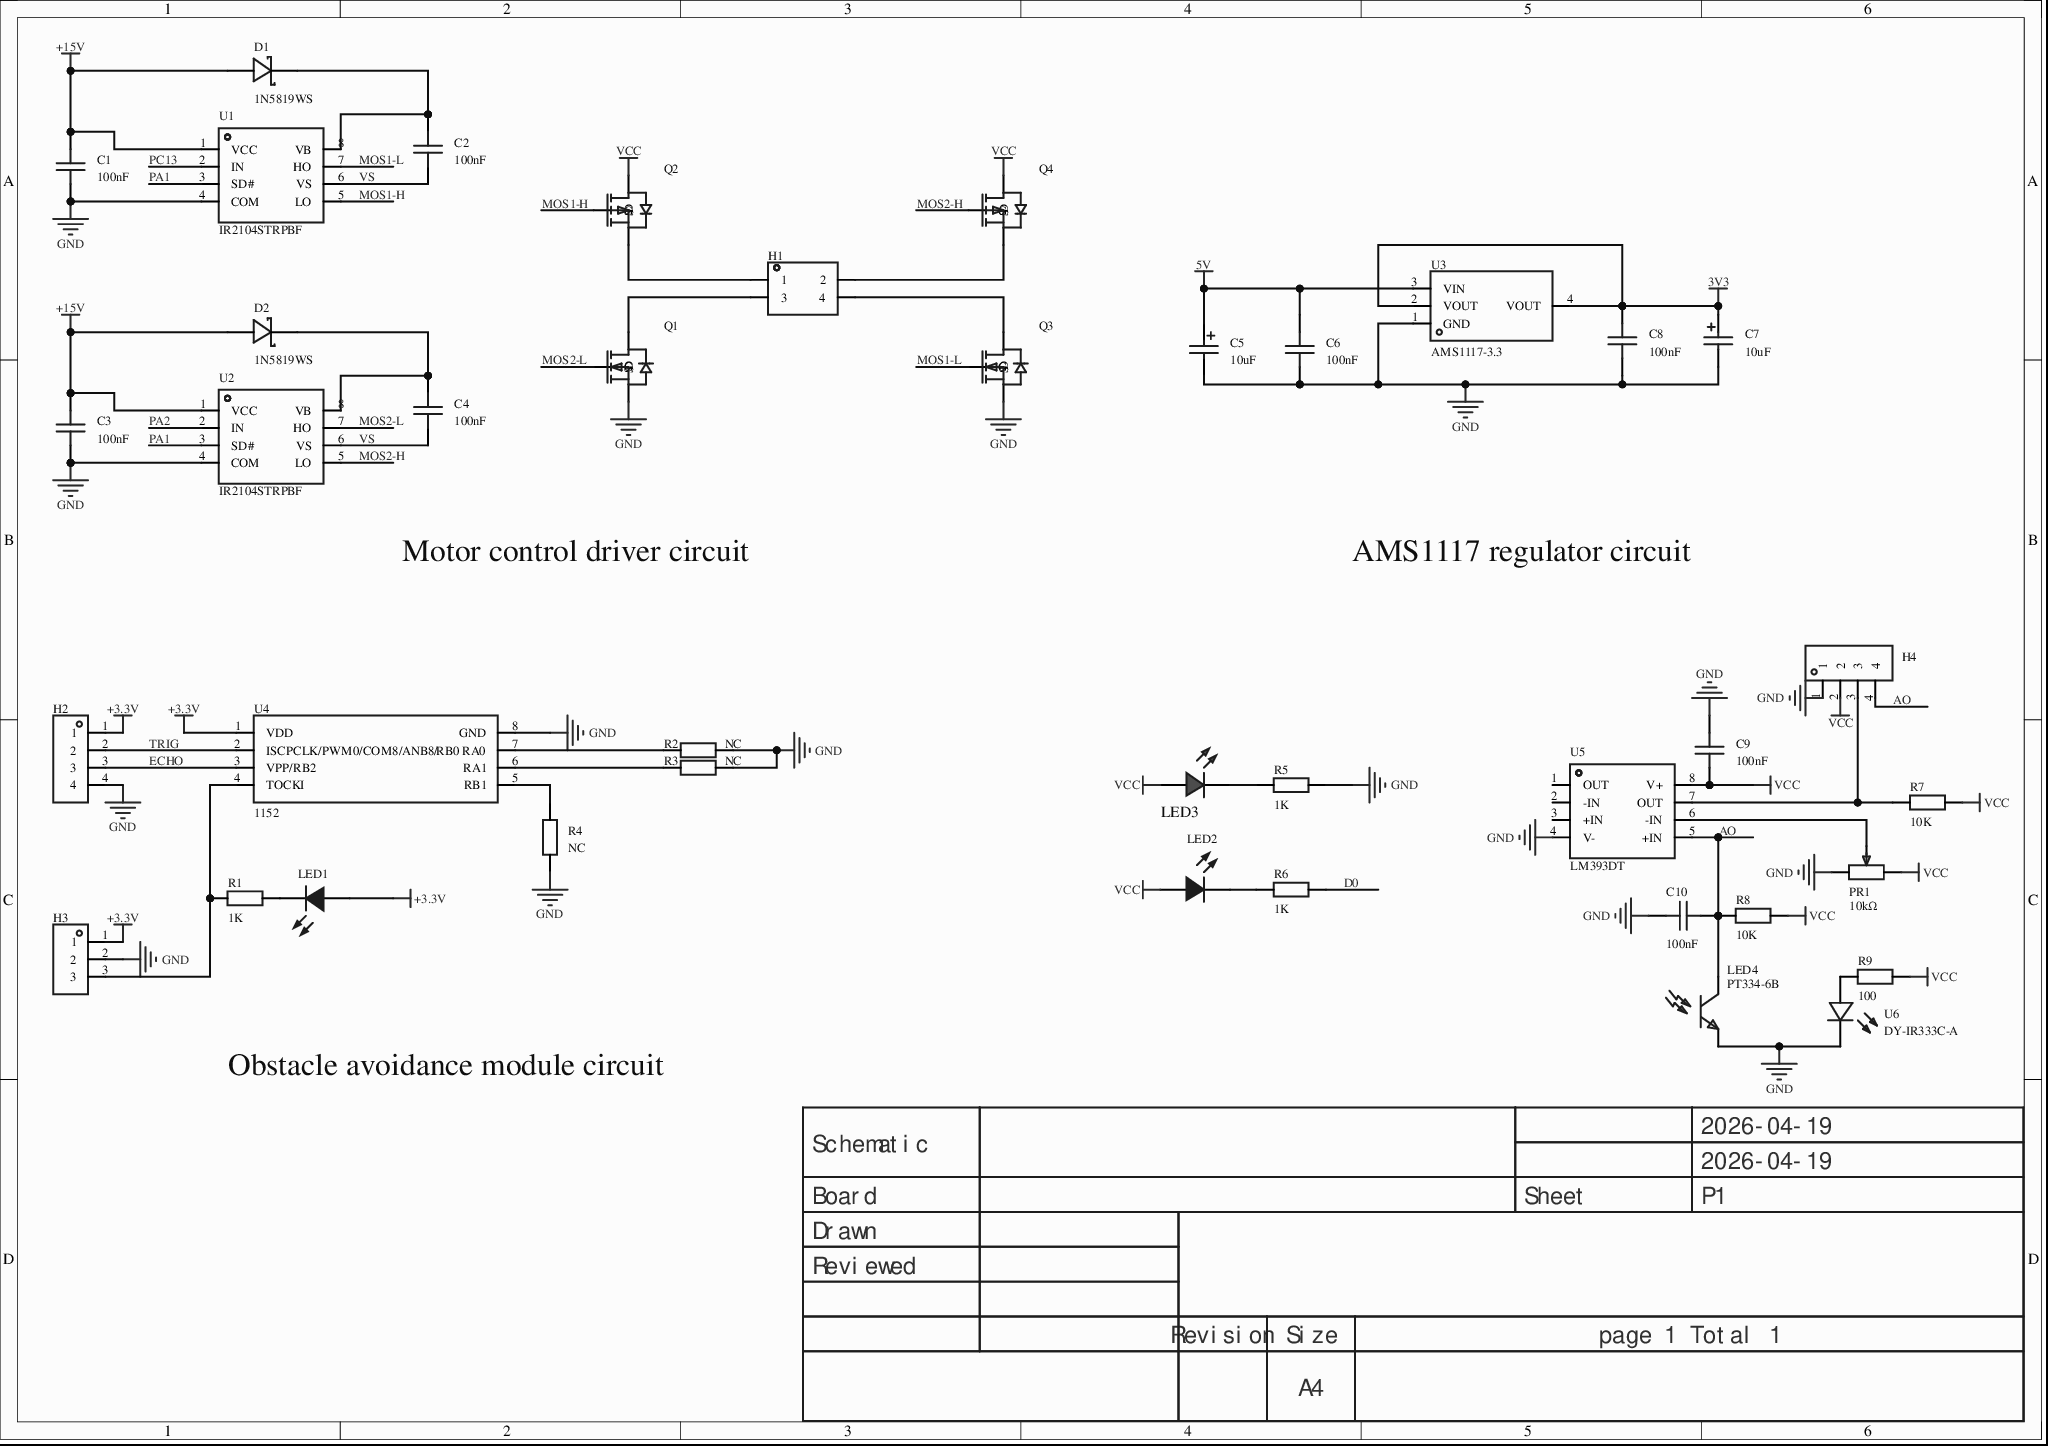
[diagram p0: MISC64784-3.schdoc]
# Altium project MISC64784-2.PrjPcb
1 sheet, 40 parts. Net scope: global (net labels, ports and power ports of the same name join across sheets).
Board file: MISC64784.pcbdoc

## Sheet MISC64784-3.schdoc
size 297 x 209 mm; Version: V1.0; @Project Name: MISC64784; @Update Date: 2026-04-19; @Create Date: 2026-04-19; @Board Name: MISC64784; @Create Time: 10:43:09; @Page Count: 1; @Page No: 1; @Schematic Name: MISC64784; @Update Time: 10:43:09; Size: A4

### Parts
C1  100nF  [C0603]
C2  100nF  [C0603]
C3  100nF  [C0603]
C4  100nF  [C0603]
C5  10uF  [C_Ele_SMD_3x5.4mm]
C6  100nF  [C0603]
C7  10uF  [C_Ele_SMD_3x5.4mm]
C8  100nF  [C0603]
C9  100nF  [C0603]
C10  100nF  [C0603]
D1  1N5819WS  [SOD-323_L1.8-W1.3-LS2.5-RD]
D2  1N5819WS  [SOD-323_L1.8-W1.3-LS2.5-RD]
H1  (no value)  [HDR-TH_4P-P2.54-V-F-R2-C2-S2.54]
H2  (no value)  [HDR-TH_4P-P2.54-V-F]
H3  (no value)  [HDR-TH_3P-P2.54-V-F]
H4  (no value)  [HDR-TH_4P-P2.54-V-M]
LED1  (no value)  [LED_0603]
LED2  (no value)  [LED_0603]
LED3  (no value)  [LED_0603]
LED4  PT334-6B  [LED-TH_BD5.9-P2.54-FD]
PR1  10kΩ  [R_3296]
Q1  (no value)  [SOT-23-3_L2.9-W1.3-P1.90-LS2.4-BR]
Q2  (no value)  [AO3401A_SOT-23-3]
Q3  (no value)  [SOT-23-3_L2.9-W1.3-P1.90-LS2.4-BR]
Q4  (no value)  [AO3401A_SOT-23-3]
R1  1K  [R0603]
R2  NC  [R0603]
R3  NC  [R0603]
R4  NC  [R0603]
R5  1K  [R0603]
R6  1K  [R0603]
R7  10K  [R0603]
R8  10K  [R0603]
R9  100  [R0603]
U1  IR2104STRPBF  [SOIC-8_L4.9-W3.9-P1.27-LS6.0-BL]
U2  IR2104STRPBF  [SOIC-8_L4.9-W3.9-P1.27-LS6.0-BL]
U3  AMS1117-3.3  [SOT-223-3_L6.5-W3.4-P2.30-LS7.0-BR]
U4  1152  [SOP-8_L4.9-W3.9-P1.27-LS6.0-BL]
U5  LM393DT  [SOIC-8_L5.0-W4.0-P1.27-LS6.0-BL]
U6  DY-IR333C-A  [LED-TH_BD5.9-P2.54-FD]

### Nets
3V3: C7.1 C8.2 U3.2(VOUT) U3.4(VOUT)
5V: C5.1 C6.2 U3.3(VIN)
+3.3V: H2.1 H3.1 LED1.2(A) U4.1(VDD)
+15V: C1.2 C3.2 D1.2(A) D2.2(A) U1.1(VCC) U2.1(VCC)
GND: C1.1 C3.1 C5.2 C6.1 C7.2 C8.1 C9.2 C10.1 H2.4 H3.2 H4.1 LED4.1(E) PR1.3 Q1.2(S) Q3.2(S) R2.2 R3.2 R4.2 R5.2 U1.4(COM) U2.4(COM) U3.1(GND) U4.8(GND) U5.4(V-) U6.2(C)
VCC: C9.1 H4.2 LED2.2(A) LED3.2(A) PR1.1 Q2.3(D) Q4.3(D) R7.2 R8.2 R9.2 U5.8(V+)
AO: C10.2 H4.4 LED4.2(C) R8.1 U5.5(+IN)
D0: R6.2
ECHO: H2.3 U4.3(VPP/RB2)
MOS1-H: Q2.1(G) U1.5(LO)
MOS1-L: Q3.1(G) U1.7(HO)
MOS2-H: Q4.1(G) U2.5(LO)
MOS2-L: Q1.1(G) U2.7(HO)
PA1: U1.3(SD#) U2.3(SD#)
PA2: U2.2(IN)
PC13: U1.2(IN)
TRIG: H2.2 U4.2(ISCPCLK/PWM0/COM8/ANB8/RB0)
VS: C2.1 C4.1 U1.6(VS) U2.6(VS)
NetC2_2: C2.2 D1.1(K) U1.8(VB)
NetC4_2: C4.2 D2.1(K) U2.8(VB)
NetH1_1: H1.1 Q2.2(S)
NetH1_2: H1.2 Q4.2(S)
NetH1_3: H1.3 Q1.3(D)
NetH1_4: H1.4 Q3.3(D)
NetH3_3: H3.3 R1.1 U4.4(TOCKI)
NetH4_3: H4.3 R7.1 U5.7(OUT)
NetLED1_1: LED1.1(C) R1.2
NetLED2_1: LED2.1(C) R6.1
NetLED3_1: LED3.1(C) R5.1
NetPR1_2: PR1.2 U5.6(-IN)
NetR2_1: R2.1 U4.7(RA0)
NetR3_1: R3.1 U4.6(RA1)
NetR4_1: R4.1 U4.5(RB1)
NetR9_1: R9.1 U6.1(A)

Not connected (* = marked no-connect by the designer): U5 1(OUT)* 2(-IN)* 3(+IN)*

### Notes on the sheet
- Motor control driver circuit
- AMS1117 regulator circuit
- Obstacle avoidance module circuit
- 2026-04-19
- Schematic
- Board
- Sheet
- P1
- Drawn
- Reviewed
- Revision
- Size
- A4
- page 1 Total 1

### Library data of the parts
C1-C4 C6 C8-C10 = CAP_0603: Symbol: Capacitance; ConvertToPcb: yes; ModelId: ac125912035d415993ca9572d50418b10819f05c4eef4c71ace90d822a990e87; ModelName: C0603_L1.6-W0.8-H0.8; ModelTransform: 62.992,31.496,0,0,0,0,0,0,0; Device: CAP_0603; AddInBom: yes; Supplier Footprint: 0603; FootprintName: C0603; Value: 100nF
C5 C7 = C_Ele_SMD_3x5.4mm: Symbol: CAP; AddInBom: yes; ModelId: 0132c3d3fdbf4fd987f710a97e7a5b5d0819f05c4eef4c71ace90d822a990e87; ModelName: CAP-SMD_BD3.0-L3.3-W3.3-H5.3; ModelTransform: 129.9,149.58,209.06,-90,0,0,0,0,0; Device: C_Ele_SMD_3x5.4mm; Supplier Footprint: SMD,3x5.4mm; ConvertToPcb: yes; FootprintName: C_Ele_SMD_3x5.4mm; Value: 10uF
D1 D2 = 1N5819WS_C191023: Forward voltage drop (Vf): 600mV@1A; DC reverse voltage (Vr): 40V; rectified current: 1A;; Manufacturer: Hottech(合科泰); AddInBom: yes; ModelId: db63db13d9e342eb939127d413d6200b0819f05c4eef4c71ace90d822a990e87; ModelTransform: 104.3305,51.181,0,0,0,0,0,-0.004,0; Non-Repetitive Peak Forward Surge Current: 25A; Symbol: 1N5819WS; Device: 1N5819WS_C191023; LCSC Part Name: 电压:40V 电流:1A; SupplierPart: C191023; ManufacturerPart: 1N5819WS; Supplier Footprint: SOD-323; JLCPCB Part Class: Basic Part; Datasheet: https://example.com/datasheet/1N5819WS/213850.html; Supplier: LCSC; ConvertToPcb: yes; FootprintName: SOD-323_L1.8-W1.3-LS2.5-RD; ModelName: SOD-323_L1.8-W1.3-LS2.5-RD; Voltage - Forward(Vf@If): 600mV@1A; Voltage - DC Reverse(Vr): 40V; Current - Rectified: 1A
H1 = HDR-F_2.54_2x2: Symbol: HDR-F-2.54_2x2; ConvertToPcb: yes; ModelId: 870c884146ee4765973edc845f10b7af0819f05c4eef4c71ace90d822a990e87; ModelName: HDR-TH_4P-P2.54-F-LI-2X2P; ModelTransform: 215.7476,196.85,0,0,0,0,0,0,-118.11; Device: HDR-F_2.54_2x2; AddInBom: yes; SupplierPart: C92273; Supplier Footprint: 插件; FootprintName: HDR-TH_4P-P2.54-V-F-R2-C2-S2.54
H2 = HDR-F_2.54_1x4P: Symbol: 2.54-1*4P female; ConvertToPcb: yes; ModelId: d187812051054f85879fcaa51a310d8e0819f05c4eef4c71ace90d822a990e87; ModelTransform: 419.6842,98.464,0,0,0,0,0,0,-118.11; Device: HDR-F_2.54_1x4P; AddInBom: yes; SupplierPart: C2718488; Supplier Footprint: 插件; FootprintName: HDR-TH_4P-P2.54-V-F; ModelName: HDR-TH_4P-P2.54-V-F
H3 = HDR-F_2.54_1x3P: Symbol: PM254V-11-03-H85; ConvertToPcb: yes; ModelId: f3b3cc5aae9641bf9e56fc160cef875b0819f05c4eef4c71ace90d822a990e87; ModelName: HDR2.54-F-LI-1X3P; ModelTransform: 299.9994,100,0,0,0,0,0,0,-118.11; Device: HDR-F_2.54_1x3P; AddInBom: yes; SupplierPart: C541850; Supplier Footprint: 插件; FootprintName: HDR-TH_3P-P2.54-V-F
H4 = HDR-M_2.54_1x4P: Symbol: PZ254V-11-04P; ConvertToPcb: yes; ModelId: 112f4d05e8d64e99ab9a333894bea4f90819f05c4eef4c71ace90d822a990e87; ModelName: HDR-TH_4P-P2.54-M-LI-1X4P; ModelTransform: 399.999,104.7242,0,0,0,0,0,0,-118.11; Device: HDR-M_2.54_1x4P; AddInBom: yes; SupplierPart: C492403; Supplier Footprint: 插件; FootprintName: HDR-TH_4P-P2.54-V-M
LED1 LED2 = LED_0603-B: Symbol: LED_B; Convert to PCB: yes; 3D Model: eb8d964598f24248affda46f619856c50819f05c4eef4c71ace90d822a990e87; 3D Model Transform: 63.1,31.6,23.7,0,0,0,0,0,0; ModelName: LED-0603_B; Device: LED_0603-B; Add into BOM: yes; Supplier Footprint: 0603; FootprintName: LED_0603
LED3 = LED_0603-R: Symbol: LED_R; Convert to PCB: yes; 3D Model: dd8257b0d61a4cd7b68939a056e080950819f05c4eef4c71ace90d822a990e87; 3D Model Transform: 58.72,29.4,22.03,0,0,0,0,0,0; ModelName: LED-0603_R; Device: LED_0603-R; Add into BOM: yes; Supplier Footprint: 0603; FootprintName: LED_0603
LED4 = PT334-6B: Transistor type: NPN; collector-emitter breakdown voltage (Vceo): 30V; collector current (Ic): 20mA; power dissipation (Pd): 75mW; dark current: 100nA; peak wavelength: 940nm;; Manufacturer: EVERLIGHT(亿光); Symbol: PT334-6B_C369188; AddInBom: yes; ModelId: 002e58ac71644a3881ed56fcedaceeee0819f05c4eef4c71ace90d822a990e87; ModelName: LED-TH_5mm_W; ModelTransform: 214.5665,231.969,0,0,0,0,-9.961,0,-137.795; Vce Saturation(VCE(sat)): 0.4V@2mA; Device: PT334-6B; LCSC Part Name: K档 940nm的NPN光电三极管; SupplierPart: C369188; ManufacturerPart: PT334-6B; Supplier Footprint: 插件,D=5mm; JLCPCB Part Class: Extended Part; Supplier: LCSC; ConvertToPcb: yes; FootprintName: LED-TH_BD5.9-P2.54-FD; type: NPN; Collector - Emitter Voltage VCEO: 30V; Current - Collector(Ic): 20mA; Dissipation Power(Max): 75mW; Current - Dark(Id): 100nA; Peak Wavelength: 940nm; Viewing Angle: -; Operating Temperature: -25℃~+85℃
PR1 = R_3296: ConvertToPcb: yes; ModelId: b182808559bb43bda9e7de64b64134cb0819f05c4eef4c71ace90d822a990e87; ModelName: 3296W; ModelTransform: 373.98,188.96,590.49,180,0,0,0,0,-140; Symbol: R_3296; Device: R_3296; AddInBom: yes; Supplier Footprint: 直插; FootprintName: R_3296; Value: 10kΩ
Q1 Q3 = AO3400A_N: 类型:N沟道;漏源电压(Vdss):30V;连续漏极电流(Id):5.2A;功率(Pd):1W;导通电阻(RDS(on)@Vgs,Id):35mΩ@10V,5A;阈值电压(Vgs(th)@Id):1.5V@250μA;; Symbol: N_MOS; AddInBom: yes; ModelId: c62791f0466c4ae2a892c056b845b0ca0819f05c4eef4c71ace90d822a990e87; ModelName: SOT-23-3P_L2.9-W1.3-H1.0-LS2.4-P0.95; ModelTransform: 98.425,114.173,0,180,0,0,0.0005,-0.0005,0; Device: AO3400A_N; Supplier Footprint: SOT-23; ConvertToPcb: yes; FootprintName: SOT-23-3_L2.9-W1.3-P1.90-LS2.4-BR; SupplierPart: C700953
Q2 Q4 = AO3401A_P: Symbol: P_MOS; AddInBom: yes; ModelId: c62791f0466c4ae2a892c056b845b0ca0819f05c4eef4c71ace90d822a990e87; ModelName: SOT-23-3P_L2.9-W1.3-H1.0-LS2.4-P0.95; ModelTransform: 98.6,114.12,41.29,180,0,0,0,0,0; Device: AO3401A_P; Supplier Footprint: SOT-23-3L; ConvertToPcb: yes; FootprintName: AO3401A_SOT-23-3; SupplierPart: C15127
R1-R9 = Res_0603: Symbol: Resistor; ConvertToPcb: yes; ModelId: fc143cca1e79419f9cd78b61e9279f080819f05c4eef4c71ace90d822a990e87; ModelTransform: 31.8897,63.7794,0,90,0,0,0,0,0; Device: Res_0603; AddInBom: yes; Supplier Footprint: 0603; FootprintName: R0603; ModelName: R0603
  R1 R5 R6: Value: 1K
  R2-R4: Value: NC
  R7 R8: Value: 10K
  R9: Value: 100
U1 U2 = IR2104STRPBF: Driver configuration: half-bridge; load type: IGBT; MOSFET; driver channels: 2; sink current (IOL): 270mA; source current (IOH): 130mA; operating voltage: 10V~20V; rise time (tr): 100ns; fall time (tf): 50ns;; Manufacturer: Infineon(英飞凌); AddInBom: yes; ModelId: e81d2f7d937b4a6ab1dca543ff5d56a40819f05c4eef4c71ace90d822a990e87; ModelName: SOIC-8_L4.9-W3.9-H1.7-LS6.0-P1.27; ModelTransform: 192.913,236.22,0,0,0,0,0,0,0; Number of Drivers: 2; Propagation Delay tpLH: 680ns; Propagation Delay tpHL: 150ns; Quiescent Current(Iq): 150uA; Symbol: IR2104STRPBF; Device: IR2104STRPBF; LCSC Part Name: 半桥驱动器; SupplierPart: C2960; ManufacturerPart: IR2104STRPBF; Supplier Footprint: SOIC-8; JLCPCB Part Class: Extended Part; Datasheet: https://example.com/datasheet/IR2104STRPBF/3342.html; Supplier: LCSC; ConvertToPcb: yes; FootprintName: SOIC-8_L4.9-W3.9-P1.27-LS6.0-BL; Driven Configuration: Half-bridge; Load Type: IGBT; MOSFET; Current - Output Low(IOL): 270mA; Current - Output High(IOH): 130mA; Voltage - Supply: 10V~20V; Rise Time: 100ns; Fall Time: 50ns; Features: Undervoltage protection (UVP); Operating Temperature: -40℃~+150℃; Input Logic Level - High: -; Input Logic Level - Low: -
U3 = AMS1117-3.3_C6186: Output type: fixed; operating voltage: 15V; output voltage: 3.3V; output current: 1A; power supply ripple rejection (PSRR): 72dB@(120Hz); output polarity: positive;; Manufacturer: AMS; AddInBom: yes; ModelId: 925194bf9823436183a3e0b978a8d0760819f05c4eef4c71ace90d822a990e87; ModelName: SOT-223-4P_L6.5-W3.5-H1.6-LS7.0-P2.30; ModelTransform: 279.89794,255.905,0,180,0,0,-3.9385,-0.0005,0; Voltage Dropout: 1.1V@(800mA); standby current: 5mA; Noise: 0.003%Vout; Number of Outputs: 1; Symbol: AMS1117-3.3; Device: AMS1117-3.3_C6186; LCSC Part Name: 3.3V 1A 15V; SupplierPart: C6186; ManufacturerPart: AMS1117-3.3; Supplier Footprint: SOT-223; JLCPCB Part Class: Basic Part; Datasheet: https://example.com/datasheet/AMS1117-3.3/6652.html; Supplier: LCSC; ConvertToPcb: yes; FootprintName: SOT-223-3_L6.5-W3.4-P2.30-LS7.0-BR; Output Type: Fixed; Voltage - Supply: 15V; Output Voltage: 3.3V; Output Current: 1A; Power Supply Rejection Ratio (PSRR): 72dB@(120Hz); Features: Overcurrent protection; thermal shutdown; Operating Temperature: -40℃~+125℃; Output Configuration: Positive
U4 = KS2505SOP8_SOP8: Symbol: KS2505SOP8_SOP8_1; AddInBom: yes; ModelId: 75c24a7891ee4dd6bdac16a7163ff87e0819f05c4eef4c71ace90d822a990e87; ModelName: SOP-8_L4.9-W3.9-P1.27-LS6.0-BL-1; ModelTransform: 192.913,236.22,0,0,0,0,0,0,0; Device: KS2505SOP8_SOP8; Manufacturer Part: 1152; LCSC Part Name: KS2505SOP8_SOP8; SupplierPart: C9900222771; Supplier Footprint: SOP8; Supplier: LCSC; ConvertToPcb: yes; FootprintName: SOP-8_L4.9-W3.9-P1.27-LS6.0-BL
U5 = LM393DT: Comparator count: dual; input offset voltage (Vos): 1mV; input bias current (Ib): 20nA;; Manufacturer: ST(意法半导体); AddInBom: yes; ModelId: 7abc64c95a1a4a04a4ef38f9097c870b0819f05c4eef4c71ace90d822a990e87; ModelTransform: 192.913,236.22,0,0,0,0,0,0,0; Propagation Delay Time: 1.3us; Output Type: TTL; MOS; DTL; CMOS; ECL; Quiescent Current: 450uA; Symbol: LM393DT; Device: LM393DT; LCSC Part Name: LM393DT; SupplierPart: C32901; ManufacturerPart: LM393DT; Supplier Footprint: SO-8; JLCPCB Part Class: Extended Part; Datasheet: https://example.com/datasheet/LM393DT/33866.html; Supplier: LCSC; ConvertToPcb: yes; FootprintName: SOIC-8_L5.0-W4.0-P1.27-LS6.0-BL; ModelName: SOIC-8_L5.0-W4.0-P1.27-LS6.0-BL; Number of Channels: Dual; Vos - Input Offset Voltage: 1mV; Ib - Input Bias Current: 20nA; Input Hysteresis Voltage (Vhys): -; Common Mode Rejection Ratio(CMRR): -; Operating Temperature: -55℃~+125℃
U6 = DY-IR333C-A_C390046: Forward voltage drop (Vf): 1.2V~1.85V; power dissipation (Pd): 150mW; wavelength: 940nm; radiant intensity: 85mW/sr; forward current: 25mA; DC reverse voltage (Vr): 5V; viewing angle: 20°;; Manufacturer: TONYU(东裕); AddInBom: yes; ModelId: 002e58ac71644a3881ed56fcedaceeee0819f05c4eef4c71ace90d822a990e87; ModelName: LED-TH_5mm_W; ModelTransform: 214.5665,231.969,0,0,0,0,-9.961,0,-137.795; Half wave width: 40nm; Symbol: DY-IR333C-A; Device: DY-IR333C-A_C390046; LCSC Part Name: F5发射管 Q等级; SupplierPart: C390046; ManufacturerPart: DY-IR333C-A; Supplier Footprint: 插件,D=5mm; JLCPCB Part Class: Extended Part; Datasheet: https://example.com/datasheet/DY-IR333C-A/366011.html; Supplier: LCSC; ConvertToPcb: yes; FootprintName: LED-TH_BD5.9-P2.54-FD; Voltage - Forward(Vf): 1.2V~1.85V; Pd - Power Dissipation: 150mW; Wavelength: 940nm; Radiant Intensity: 85mW/sr; Current - DC Forward(If): 25mA; Voltage - DC Reverse(Vr): 5V; Viewing Angle: 20°; Operating Temperature: -25℃~+80℃